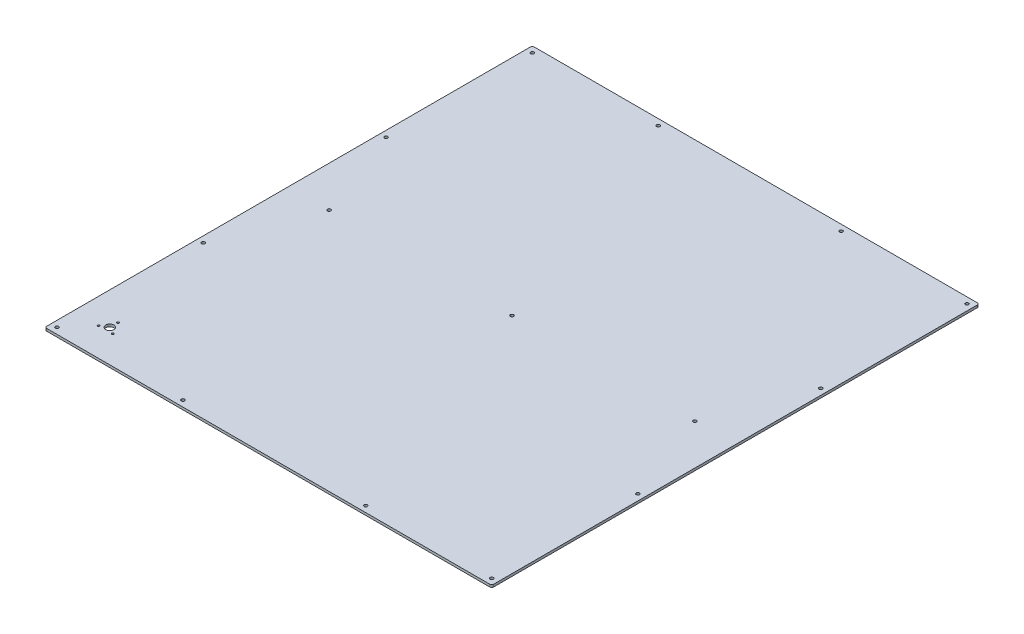
from build123d import *

# Parameters (mm, degrees)
SKETCH_1_W            = 1100
SKETCH_1_H            = 1200
EXTRUDE_1_DEPTH       = 6
FILLET_1_R            = 5
HOLE_WIZARD_8_0_8_1_D = 8
SKETCH_4_R            = 10
CUT_EXTRUDE_1_DEPTH   = 814.963144129
HOLE_WIZARD_5_0_5_1_D = 5


with BuildPart() as part:
    # 草图1 → 凸台-拉伸1 (new body)
    with BuildSketch(Plane(origin=(0, 0, 0), x_dir=(1, 0, 0), z_dir=(0, 1, 0))):
        Rectangle(SKETCH_1_W, SKETCH_1_H)
    extrude(amount=EXTRUDE_1_DEPTH)

    # 圆角1
    fillet_1_edges = [part.edges().sort_by_distance(p)[0] for p in [
        (550, 3, 600),
        (-550, 3, 600),
        (-550, 3, -600),
        (550, 3, -600),
    ]]
    fillet(fillet_1_edges, radius=FILLET_1_R)

    # Ø8.0 (8) 直径孔1 (through all)
    with Locations(Plane(origin=(0, 6, 0), x_dir=(1, 0, 0), z_dir=(0, 1, 0))):
        with Locations((-535, 585), (535, 585), (-535, -585), (535, -585), (-225, -585), (225, -585), (0, 0), (-225, 585), (225, 585), (-535, -225), (-535, 225), (535, 225), (535, -225), (-450, 0), (450, 0)):
            Hole(HOLE_WIZARD_8_0_8_1_D / 2)

    # 草图4 → 切除-拉伸1 (cut, through all)
    with BuildSketch(Plane(origin=(0, 6, 0), x_dir=(1, 0, 0), z_dir=(0, 1, 0))):
        with Locations(Location((-470, -520, 0), (0, 0, 270))):
            Circle(SKETCH_4_R)
    extrude(amount=-CUT_EXTRUDE_1_DEPTH, mode=Mode.SUBTRACT)

    # Ø5.0 (5) 直径孔1 (through all)
    with Locations(Plane(origin=(0, 6, 0), x_dir=(1, 0, 0), z_dir=(0, 1, 0))):
        with Locations((-470, -499.792740578), (-452.5, -530.103629711), (-487.5, -530.103629711)):
            Hole(HOLE_WIZARD_5_0_5_1_D / 2)


solid = part.part
